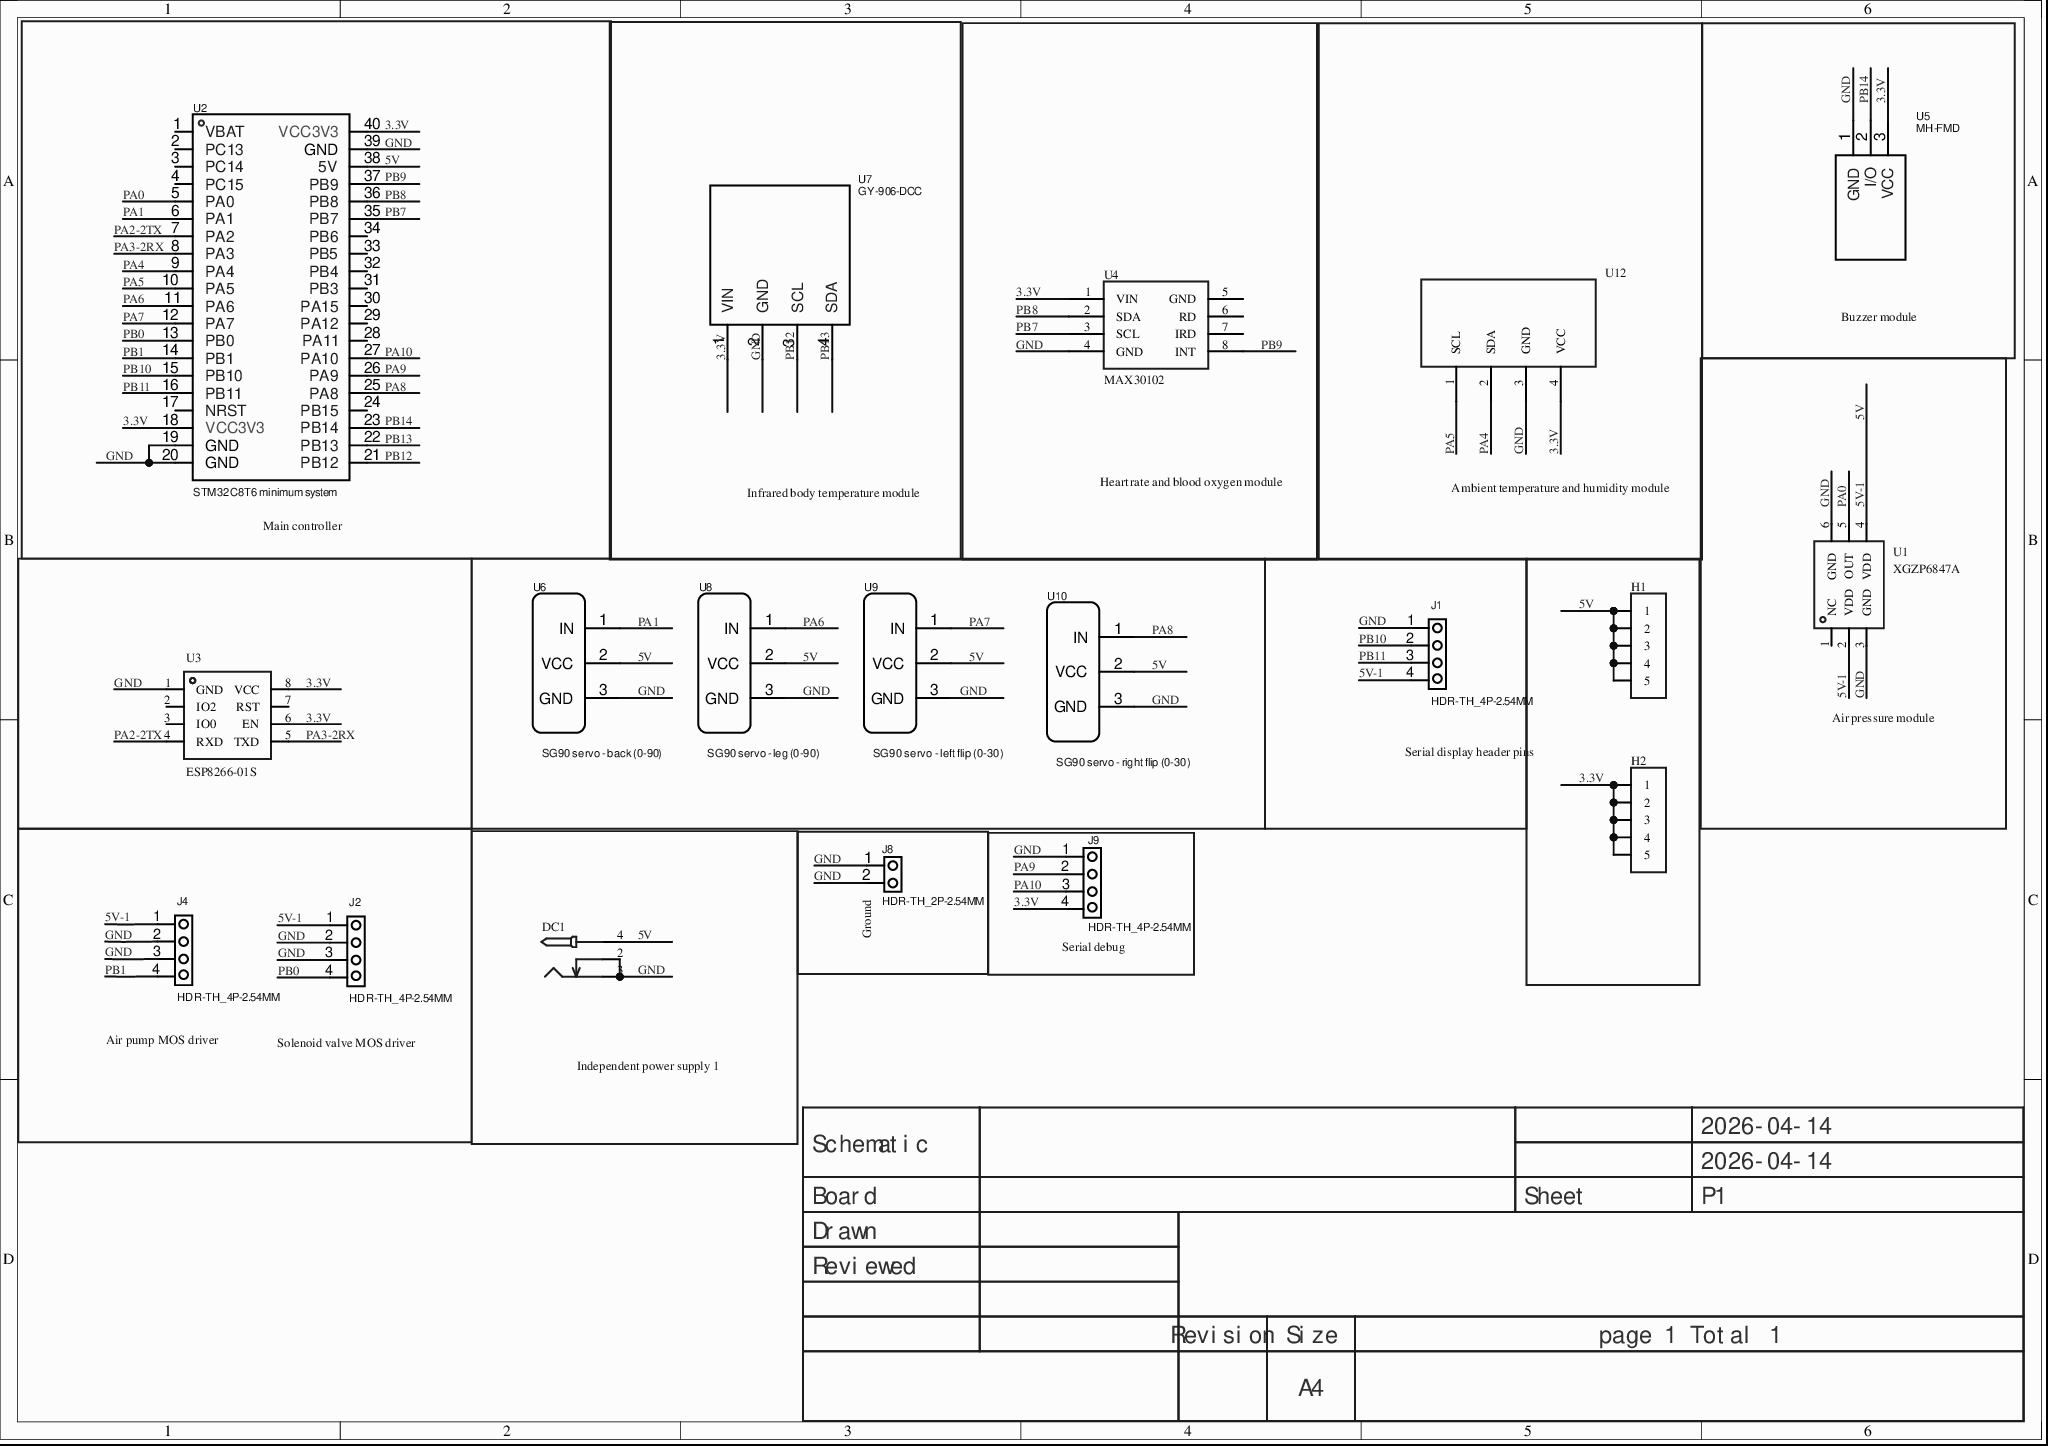
[diagram p0: MISC51766-3.schdoc]
# Altium project MISC51766-2.PrjPcb
1 sheet, 19 parts. Net scope: global (net labels, ports and power ports of the same name join across sheets).
Board file: MISC51766.pcbdoc

## Sheet MISC51766-3.schdoc
size 297 x 209 mm; Version: V1.0; @Project Name: MISC51766; @Update Date: 2026-04-14; @Create Date: 2026-04-14; @Board Name: MISC51766; @Create Time: 11:59:48; @Page Count: 1; @Page No: 1; @Schematic Name: MISC51766; @Update Time: 11:59:48; Size: A4

### Parts
DC1  (no value)  [DC-2.0]
H1  (no value)  [HDR-TH_5P-P2.54-V-F]
H2  (no value)  [HDR-TH_5P-P2.54-V-F]
J1  HDR-TH_4P-2.54MM  [HDR-TH_4P-2.54MM]
J2  HDR-TH_4P-2.54MM  [HDR-TH_4P-2.54MM]
J4  HDR-TH_4P-2.54MM  [HDR-TH_4P-2.54MM]
J8  HDR-TH_2P-2.54MM  [HDR-TH_2P-2.54MM]
J9  HDR-TH_4P-2.54MM  [HDR-TH_4P-2.54MM]
U1  XGZP6847A  [SENSOR-TH_XGZP6847A]
U2  STM32C8T6 minimum system  [STM32F103C8T6最小系统插座]
U3  ESP8266-01S  [WIFIM-TH_ESP8266-01S]
U4  MAX30102  [MAX30102]
U5  MH-FMD  [MH-FMD]
U6  SG90 servo - back (0-90)  [SG90]
U7  GY-906-DCC  [GY-906-DCC]
U8  SG90 servo - leg (0-90)  [SG90]
U9  SG90 servo - left flip (0-30)  [SG90]
U10  SG90 servo - right flip (0-30)  [SG90]
U12  (no value)  [SHT30]

### Blocks framed on the sheet
Main controller: U2
Infrared body temperature module: U7
Heart rate and blood oxygen module: U4
Ambient temperature and humidity module: U12
Buzzer module: U5
Air pressure module: U1
Serial display header pins: J1
Independent power supply 1: DC1
Ground: J8
Serial debug: J9

### Nets
3.3V: H2.1 H2.2 H2.3 H2.4 H2.5 J9.4 U2.18(VCC3V3) U2.40(VCC3V3) U3.6(EN) U3.8(VCC) U4.1(VIN) U5.3(VCC) U7.1(VIN) U12.4(VCC)
5V: DC1.4 H1.1 H1.2 H1.3 H1.4 H1.5 J1.4 J2.1 J4.1 U1.2(VDD) U1.4(VDD) U2.38(5V) U6.2(VCC) U8.2(VCC) U9.2(VCC) U10.2(VCC)  [also labelled 5V-1]
GND: DC1.2 DC1.3 J1.1 J2.2 J2.3 J4.2 J4.3 J8.1 J8.2 J9.1 U1.3(GND) U1.6(GND) U2.19(GND) U2.20(GND) U2.39(GND) U3.1(GND) U4.4(GND) U5.1(GND) U6.3(GND) U7.2(GND) U8.3(GND) U9.3(GND) U10.3(GND) U12.3(GND)
PA0: U1.5(OUT) U2.5(PA0)
PA1: U2.6(PA1) U6.1(IN)
PA2-2TX: U2.7(PA2) U3.4(RXD)
PA3-2RX: U2.8(PA3) U3.5(TXD)
PA4: U2.9(PA4) U12.2(SDA)
PA5: U2.10(PA5) U12.1(SCL)
PA6: U2.11(PA6) U8.1(IN)
PA7: U2.12(PA7) U9.1(IN)
PA8: U2.25(PA8) U10.1(IN)
PA9: J9.2 U2.26(PA9)
PA10: J9.3 U2.27(PA10)
PB0: J2.4 U2.13(PB0)
PB1: J4.4 U2.14(PB1)
PB7: U2.35(PB7) U4.3(SCL)
PB8: U2.36(PB8) U4.2(SDA)
PB9: U2.37(PB9) U4.8(INT)
PB10: J1.2 U2.15(PB10)
PB11: J1.3 U2.16(PB11)
PB12: U2.21(PB12) U7.3(SCL)
PB13: U2.22(PB13) U7.4(SDA)
PB14: U2.23(PB14) U5.2(I/O)

Not connected (* = marked no-connect by the designer): U1 1(NC)*; U2 1(VBAT)* 2(PC13)* 3(PC14)* 4(PC15)* 17(NRST)* 24(PB15)* 28(PA11)* 29(PA12)* 30(PA15)* 31(PB3)* 32(PB4)* 33(PB5)* 34(PB6)*; U3 2(IO2)* 3(IO0)* 7(RST)*; U4 5(GND)* 6(RD)* 7(IRD)*

### Notes on the sheet
- (near J4) Air pump MOS driver
- (near J2) Solenoid valve MOS driver
- 2026-04-14
- Schematic
- Board
- Sheet
- P1
- Drawn
- Reviewed
- Revision
- Size
- A4
- page 1 Total 1

### Library data of the parts
DC1 = DC-005_2.0: Symbol: DC power connector; ConvertToPcb: yes; ModelId: f5f20b8a2308479b936ba3c2698865bb0819f05c4eef4c71ace90d822a990e87; ModelName: DC-IN-TH_DC-5520-1; ModelTransform: 372.05,551.18,582.68,90,0,0,137.8,0,-149.61; Device: DC-005_2.0; AddInBom: yes; Supplier Footprint: 插件; FootprintName: DC-2.0
H1 H2 = HDR-F_2.54_1x5P: Symbol: Header-Female-2.54_1x5; ConvertToPcb: yes; ModelId: f49cb6116a3d45e5a64915bf3e00773f0819f05c4eef4c71ace90d822a990e87; ModelTransform: 519.684,98.464,0,0,0,0,0,0,-124.016; Device: HDR-F_2.54_1x5P; AddInBom: yes; SupplierPart: C50950; Supplier Footprint: 插件; FootprintName: HDR-TH_5P-P2.54-V-F; ModelName: HDR-TH_5P-P2.54-V-F
U1 = XGZP6847A: AddInBom: yes; ModelId: 62bfc9b7d7f74308aff708257f1a458b0819f05c4eef4c71ace90d822a990e87; ModelTransform: 511.81,511.81,0,180,0,0,0,0,-137.795; Symbol: XGZP6847A; Device: XGZP6847A; LCSC Part Name: XGZP6847A; SupplierPart: C9900001043; ManufacturerPart: XGZP6847A; Supplier Footprint: TH-6_13.0X13.0X2.54P; JLCPCB Part Class: Extended Part; Supplier: LCSC; ConvertToPcb: yes; FootprintName: SENSOR-TH_XGZP6847A; ModelName: SENSOR-TH_XGZP6847A
U2 = STM32C8T6最小系统: Symbol: STM32C8T6 minimum system; Device: STM32C8T6 minimum system; FootprintName: STM32F103C8T6 minimum system socket
U3 = ESP8266-01S: AddInBom: yes; ModelId: 7671a3a19d0d4245ae5d5806b59f4d510819f05c4eef4c71ace90d822a990e87; ModelTransform: 566.928,972.439,0,0,0,0,0,378.464,-118.11; Symbol: ESP8266-01S; Device: ESP8266-01S; LCSC Part Name: ESP8266-01S; SupplierPart: C9900150497; ManufacturerPart: ESP8266-01S; Supplier Footprint: TH-8P; JLCPCB Part Class: Extended Part; Supplier: LCSC; ConvertToPcb: yes; FootprintName: WIFIM-TH_ESP8266-01S; ModelName: WIFIM-TH_ESP8266-01S
U4 = MAX30102: AddInBom: yes; Symbol: MAX30102; Device: MAX30102; ConvertToPcb: yes; FootprintName: MAX30102
U6 U8-U10 = SG90舵机: Symbol: SG90 servo; Device: SG90 servo; FootprintName: SG90
  U6 U8 U9: OriginFootprint: SG90
  U10: Origin Footprint: SG90
U7 = GY-906-DCC: description: Long-range infrared temperature detection module for body temperature monitoring; Symbol: GY-906-DCC; Device: GY-906-DCC; FootprintName: GY-906-DCC
U12 = SHT30: AddInBom: yes; Symbol: SHT30; Device: SHT30; ConvertToPcb: yes; FootprintName: SHT30
J1 J2 J4 J9 = HDR-TH_4P-2.54MM: Symbol: HDR-TH_4P-2.54MM; Device: HDR-TH_4P-2.54MM; SupplierPart: HDR-TH_4P-2.54MM; Supplier: LCSC; Manufacturer: HDR-TH_4P-2.54MM; ManufacturerPart: HDR-TH_4P-2.54MM; link: HDR-TH_4P-2.54MM; OriginFootprint: HDR-TH_4P-2.54MM; FootprintName: HDR-TH_4P-2.54MM; supplierPart: HDR-TH_4P-2.54MM; manufacturer: HDR-TH_4P-2.54MM
J8 = HDR-TH_2P-2.54MM: Symbol: HDR-TH_2P-2.54MM; Device: HDR-TH_2P-2.54MM; SupplierPart: HDR-TH_2P-2.54MM; Supplier: LCSC; Manufacturer: HDR-TH_2P-2.54MM; ManufacturerPart: HDR-TH_2P-2.54MM; link: HDR-TH_2P-2.54MM; OriginFootprint: HDR-TH_2P-2.54MM; FootprintName: HDR-TH_2P-2.54MM; supplierPart: HDR-TH_2P-2.54MM; manufacturer: HDR-TH_2P-2.54MM; description: HDR-TH_2P-2.54MM
U5 = MH-FMD: Symbol: MH-FMD; Device: MH-FMD; OriginFootprint: MH-FMD; FootprintName: MH-FMD